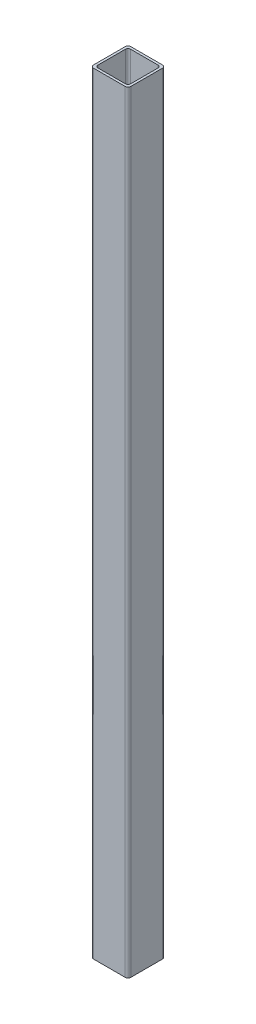
from build123d import *

# Parameters (mm, degrees)
BOSS_EXTRUDE1_DEPTH = 2070


with BuildPart() as part:
    # Sketch2 → Boss-Extrude1 (new body)
    with BuildSketch(Plane(origin=(0, 0, 0), x_dir=(1, 0, 0), z_dir=(0, 1, 0))):
        with BuildLine():
            Line((7.875, -1.525), (92.125, -1.525))
            ThreePointArc((92.125, -1.525), (97.693465902, 0.781534098), (100, 6.35))
            Line((100, 6.35), (100, 90.6))
            ThreePointArc((100, 90.6), (97.693465902, 96.168465902), (92.125, 98.475))
            Line((92.125, 98.475), (7.875, 98.475))
            ThreePointArc((7.875, 98.475), (2.306534098, 96.168465902), (0, 90.6))
            Line((0, 90.6), (0, 6.35))
            ThreePointArc((0, 6.35), (2.306534098, 0.781534098), (7.875, -1.525))
        make_face()
        with BuildLine():
            Line((12.6, 4.775), (87.4, 4.775))
            ThreePointArc((87.4, 4.775), (91.854772721, 6.620227279), (93.7, 11.075))
            Line((93.7, 11.075), (93.7, 85.875))
            ThreePointArc((93.7, 85.875), (91.854772721, 90.329772721), (87.4, 92.175))
            Line((87.4, 92.175), (12.6, 92.175))
            ThreePointArc((12.6, 92.175), (8.145227279, 90.329772721), (6.3, 85.875))
            Line((6.3, 85.875), (6.3, 11.075))
            ThreePointArc((6.3, 11.075), (8.145227279, 6.620227279), (12.6, 4.775))
        make_face(mode=Mode.SUBTRACT)
    extrude(amount=BOSS_EXTRUDE1_DEPTH)


solid = part.part
